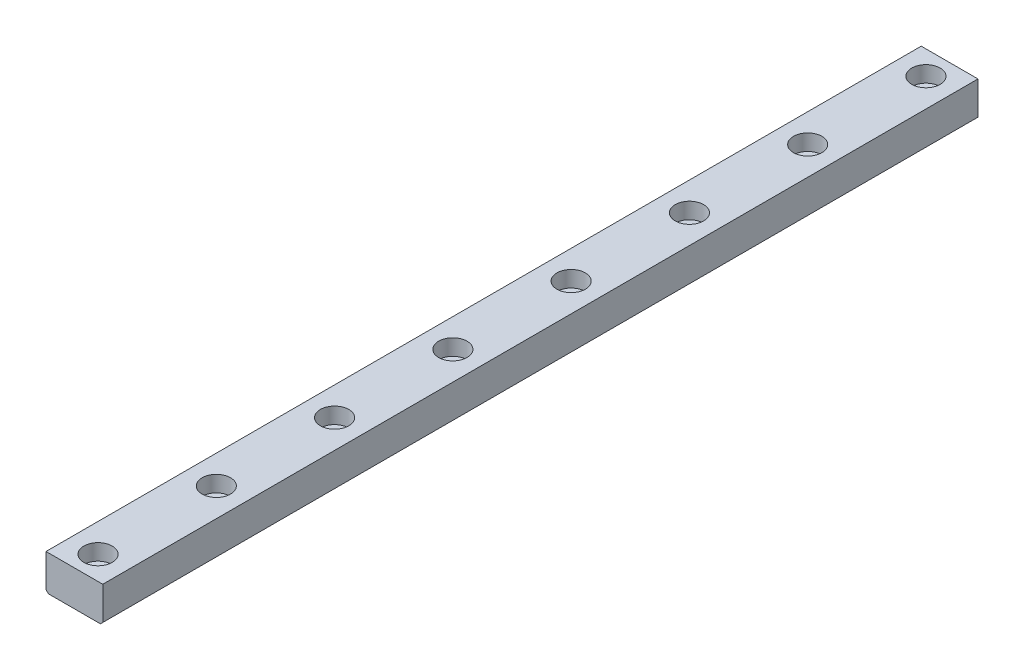
from build123d import *

# Parameters (mm, degrees)
SKETCH1_W                                            = 12
SKETCH1_H                                            = 7.5
BOSS_EXTRUDE1_DEPTH                                  = 185
CHAMFER1_SIZE                                        = 0.5
HOLE_SIZE_PER_SOCKET_HEAD_CAP_SCREW_TYPE_D           = 3.4
HOLE_SIZE_PER_SOCKET_HEAD_CAP_SCREW_TYPE_CBORE_D     = 6
HOLE_SIZE_PER_SOCKET_HEAD_CAP_SCREW_TYPE_CBORE_DEPTH = 3.4
LPATTERN1_COUNT                                      = 8
LPATTERN1_PITCH                                      = 25


with BuildPart() as part:
    # Sketch1 → Boss-Extrude1 (new body)
    with BuildSketch(Plane.XY):
        Rectangle(SKETCH1_W, SKETCH1_H)
    extrude(amount=BOSS_EXTRUDE1_DEPTH)

    # Chamfer1
    chamfer1_edges = [part.edges().sort_by_distance(p)[0] for p in [
        (6, -3.75, 92.5),
        (-6, -3.75, 92.5),
    ]]
    chamfer(chamfer1_edges, length=CHAMFER1_SIZE)

    # Hole size per socket head cap screw type1 (through all)
    with Locations(Plane(origin=(0, 3.75, 0), x_dir=(-1, 0, 0), z_dir=(0, 1, 0))):
        with Locations((0, 5)):
            hole_size_per_socket_head_cap_screw_type = CounterBoreHole(HOLE_SIZE_PER_SOCKET_HEAD_CAP_SCREW_TYPE_D / 2, HOLE_SIZE_PER_SOCKET_HEAD_CAP_SCREW_TYPE_CBORE_D / 2, HOLE_SIZE_PER_SOCKET_HEAD_CAP_SCREW_TYPE_CBORE_DEPTH)

    # LPattern1: Hole size per socket head cap screw type1 ×8
    with Locations(*[(0, 0, i * LPATTERN1_PITCH) for i in range(1, LPATTERN1_COUNT)]):
        add(hole_size_per_socket_head_cap_screw_type, mode=Mode.SUBTRACT)


solid = part.part
